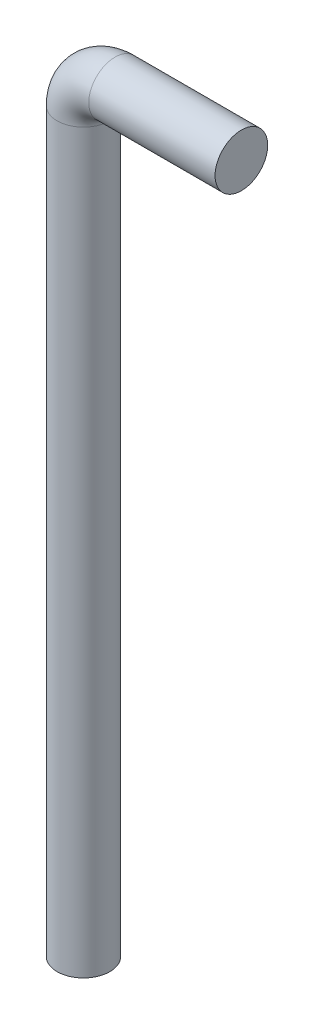
SolidWorks part; units mm, degrees
ref_plane "前视基准面" through (0, 0, 0) normal (0, 0, 1) x (1, 0, 0)
ref_plane "上视基准面" through (0, 0, 0) normal (0, 1, 0) x (1, 0, 0)
ref_plane "右视基准面" through (0, 0, 0) normal (1, 0, 0) x (0, 0, -1)
sketch "草图16" plane through (0, 0, 0) normal (0, 1, 0) x (1, 0, 0)
  circle A0 centre (0, 0) radius 2.5
  dimension "D1" = 5
sketch "草图17" plane through (0, 0, 0) normal (0, 0, 1) x (1, 0, 0)
  line L0 (0, 0) -> (0, 70)
  line L1 (3, 73) -> (15, 73)
  arc A0 (0, 70) -> (3, 73) centre (3, 70) cw
  point P6 (0, 73)
  dimension "D3" = 3
  dimension "D1" = 73
  dimension "D2" = 15
sweep "扫描1" add profiles "草图16" path "草图17"
